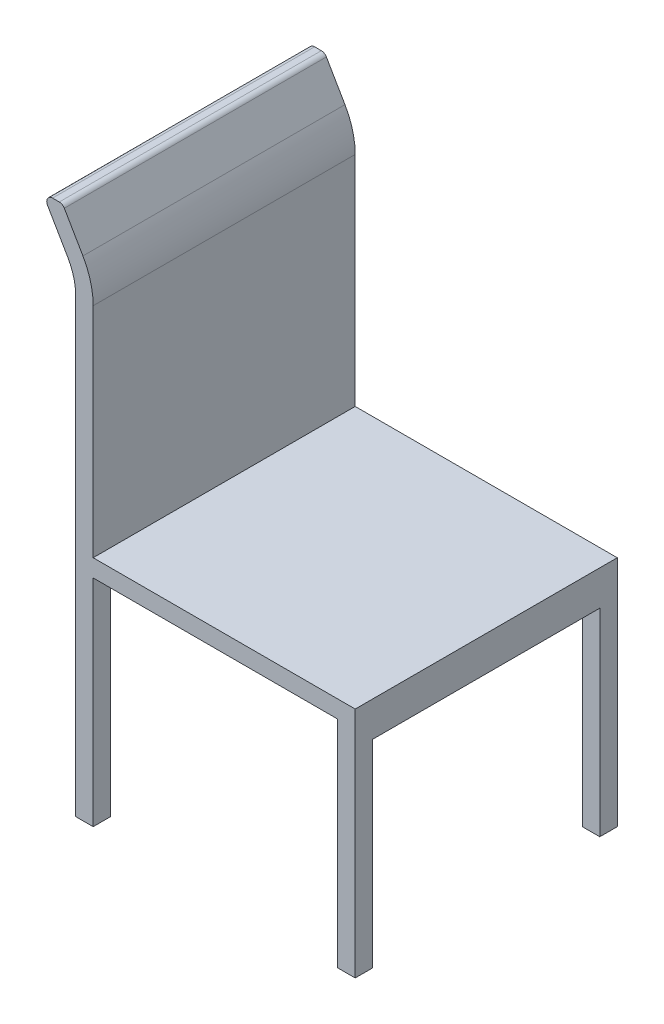
SolidWorks part; units mm, degrees
material "红木"
ref_plane "Front Plane" through (0, 0, 0) normal (0, 0, 1) x (1, 0, 0)
ref_plane "Top Plane" through (0, 0, 0) normal (0, 1, 0) x (1, 0, 0)
ref_plane "Right Plane" through (0, 0, 0) normal (1, 0, 0) x (0, 0, -1)
sketch "Sketch1" plane through (0, 0, 0) normal (0, 0, 1) x (1, 0, 0)
  line L0 (0, 0) -> (0, 774.7618)
  line L2 (-28.1408, 900) -> (-39.7035, 900)
  line L3 (30, 400) -> (480, 400)
  line L4 (480, 400) -> (480, 0)
  line L5 (480, 0) -> (450, 0)
  line L6 (450, 0) -> (450, 370)
  line L7 (450, 370) -> (30, 370)
  line L8 (30, 370) -> (30, 0)
  line L9 (30, 0) -> (0, 0)
  line L10 (-13.5146, 824.9641) -> (-48.352, 884.9798)
  line L11 (12.431, 840.0249) -> (-19.4923, 895.0202)
  line L12 (30, 774.7618) -> (30, 400)
  line L13 (55.9456, 765.0607) -> (-21.8001, 898.9959) construction
  line L14 (30, 750) -> (-47.7457, 883.9352) construction
  arc A0 (0, 774.7618) -> (-13.5146, 824.9641) centre (-100, 774.7618) ccw
  arc A1 (12.431, 840.0249) -> (30, 774.7618) centre (-100, 774.7618) cw
  arc A2 (-19.4923, 895.0202) -> (-28.1408, 900) centre (-28.1408, 890) ccw
  arc A3 (-48.352, 884.9798) -> (-39.7035, 900) centre (-39.7035, 890) cw
  dimension "D1" = 100
  dimension "D4" = 130
  dimension "D8" = 10
  dimension "D2" = 450
  dimension "D3" = 420
  dimension "D5" = 30
  dimension "D6" = 370
  dimension "D7" = 400
  dimension "D9" = 30
extrude "Boss-Extrude1" add sketch "Sketch1" along normal blind 450
sketch "Sketch2" plane through (480, 0, 0) normal (1, 0, 0) x (0, 0, -1)
  line L0 (-450, 400) -> (0, 400) construction
  line L1 (-420, 340) -> (-30, 340)
  line L2 (-420, 340) -> (-420, -25.7975)
  line L3 (-420, -25.7975) -> (-30, -25.7975)
  line L4 (-30, 340) -> (-30, -25.7975)
  line L5 (-450, 0) -> (-450, 400) construction
  line L6 (0, 0) -> (0, 400) construction
  dimension "D1" = 60
  dimension "D2" = 30
  dimension "D3" = 30
extrude "Cut-Extrude1" cut sketch "Sketch2" against normal blind 500
